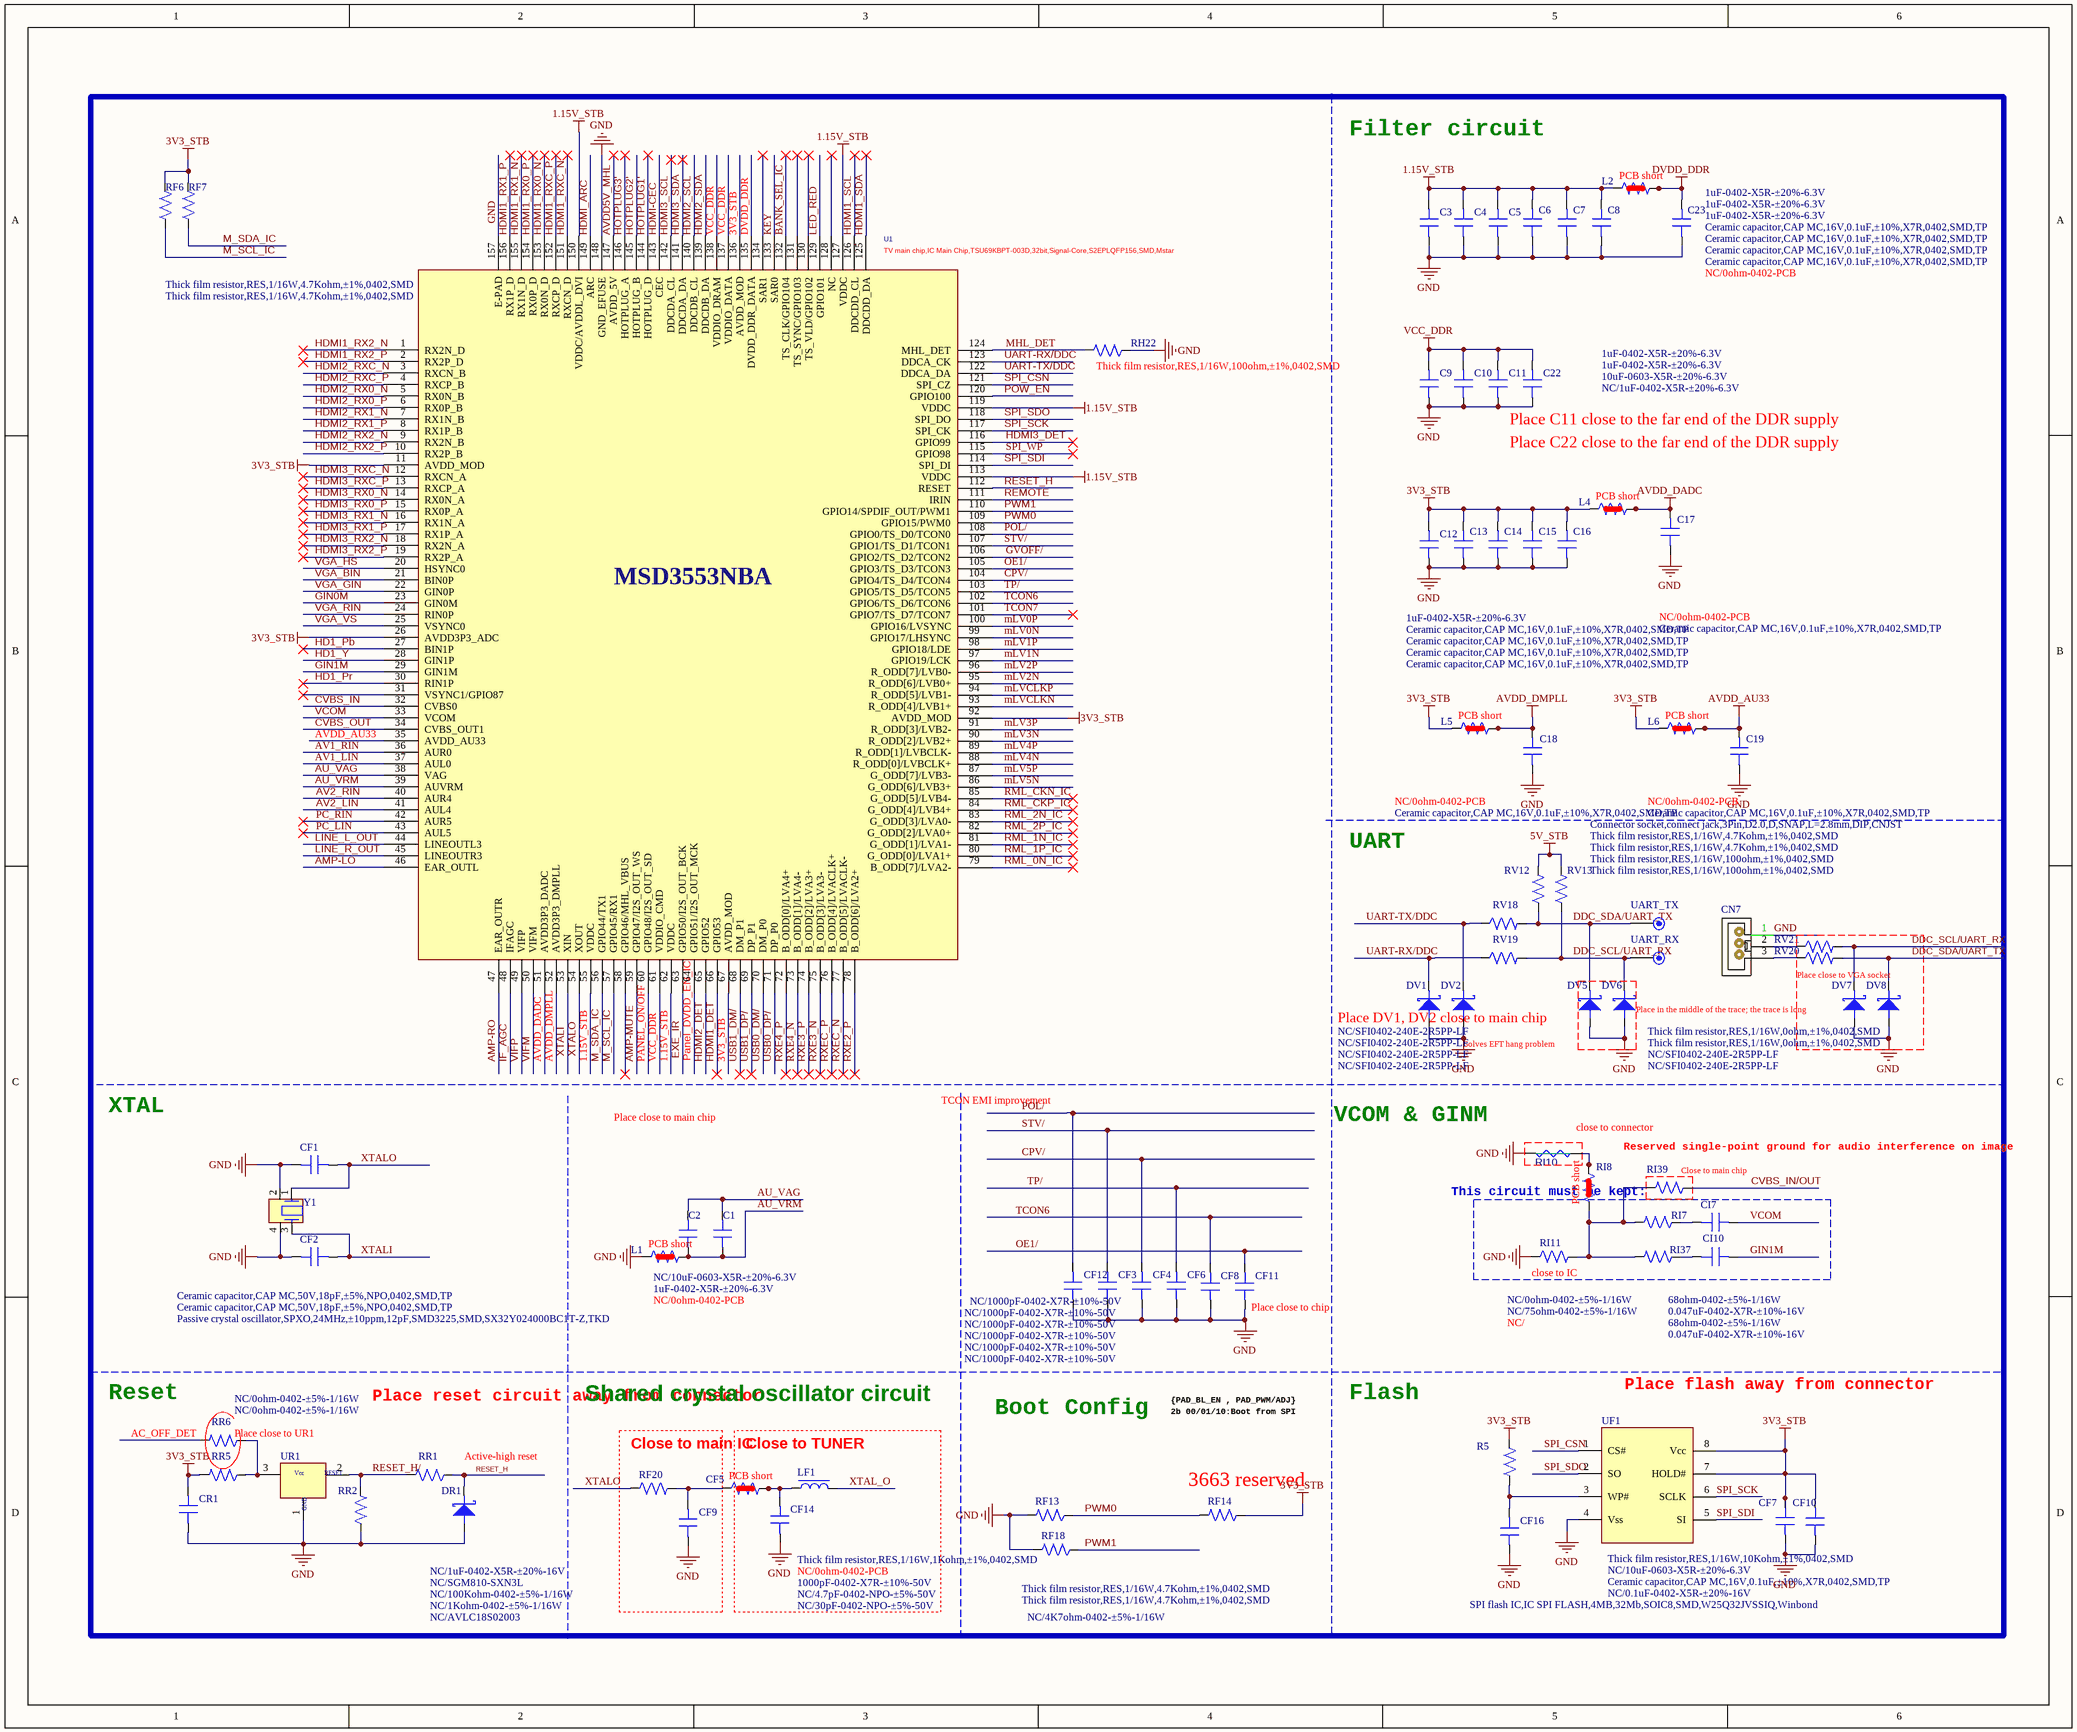
[diagram p0: MISC86383-12.SchDoc]
# Altium project MISC86383-33.PrjPCB (part 2 of 8)

## Sheet MISC86383-12.SchDoc
size 457 x 381 mm

### Parts
C1  1uF-0402-X5R-±20%-6.3V  [C0402]
C2  NC/10uF-0603-X5R-±20%-6.3V  [C0603]
C3  1uF-0402-X5R-±20%-6.3V  [C0402]
C4  1uF-0402-X5R-±20%-6.3V  [C0402]
C5  1uF-0402-X5R-±20%-6.3V  [C0402]
C6  Ceramic capacitor,CAP MC,16V,0.1uF,±10%,X7R,0402,SMD,TP  [C0402]
C7  Ceramic capacitor,CAP MC,16V,0.1uF,±10%,X7R,0402,SMD,TP  [C0402]
C8  Ceramic capacitor,CAP MC,16V,0.1uF,±10%,X7R,0402,SMD,TP  [C0402]
C9  1uF-0402-X5R-±20%-6.3V  [C0402]
C10  1uF-0402-X5R-±20%-6.3V  [C0402]
C11  10uF-0603-X5R-±20%-6.3V  [C0603]
C12  1uF-0402-X5R-±20%-6.3V  [C0402]
C13  Ceramic capacitor,CAP MC,16V,0.1uF,±10%,X7R,0402,SMD,TP  [C0402]
C14  Ceramic capacitor,CAP MC,16V,0.1uF,±10%,X7R,0402,SMD,TP  [C0402]
C15  Ceramic capacitor,CAP MC,16V,0.1uF,±10%,X7R,0402,SMD,TP  [C0402]
C16  Ceramic capacitor,CAP MC,16V,0.1uF,±10%,X7R,0402,SMD,TP  [C0402]
C17  Ceramic capacitor,CAP MC,16V,0.1uF,±10%,X7R,0402,SMD,TP  [C0402]
C18  Ceramic capacitor,CAP MC,16V,0.1uF,±10%,X7R,0402,SMD,TP  [C0402]
C19  Ceramic capacitor,CAP MC,16V,0.1uF,±10%,X7R,0402,SMD,TP  [C0402]
C22  NC/1uF-0402-X5R-±20%-6.3V  [C0402]
C23  Ceramic capacitor,CAP MC,16V,0.1uF,±10%,X7R,0402,SMD,TP  [C0402]
CF1  Ceramic capacitor,CAP MC,50V,18pF,±5%,NPO,0402,SMD,TP  [C0402]
CF2  Ceramic capacitor,CAP MC,50V,18pF,±5%,NPO,0402,SMD,TP  [C0402]
CF3  NC/1000pF-0402-X7R-±10%-50V  [C0402]
CF4  NC/1000pF-0402-X7R-±10%-50V  [C0402]
CF5  NC/0ohm-0402-PCB  [R0402SC]
CF6  NC/1000pF-0402-X7R-±10%-50V  [C0402]
CF7  Ceramic capacitor,CAP MC,16V,0.1uF,±10%,X7R,0402,SMD,TP  [C0402]
CF8  NC/1000pF-0402-X7R-±10%-50V  [C0402]
CF9  NC/30pF-0402-NPO-±5%-50V  [C0402]
CF10  NC/10uF-0603-X5R-±20%-6.3V  [C0603]
CF11  NC/1000pF-0402-X7R-±10%-50V  [C0402]
CF12  NC/1000pF-0402-X7R-±10%-50V  [C0402]
CF14  NC/4.7pF-0402-NPO-±5%-50V  [C0402]
CF16  NC/0.1uF-0402-X5R-±20%-16V  [C0402]
CI7  0.047uF-0402-X7R-±10%-16V  [C0402]
CI10  0.047uF-0402-X7R-±10%-16V  [C0402]
CN7  Connector socket,connect jack,3Pin,D2.0,D,SNAP,L=2.8mm,DIP,CNJST  [SIP3/2.0D-3]
CR1  NC/1uF-0402-X5R-±20%-16V  [C0402]
DR1  NC/AVLC18S02003  [DIODE-S0402]
DV1  NC/SFI0402-240E-2R5PP-LF  [DIODE-S0402]
DV2  NC/SFI0402-240E-2R5PP-LF  [DIODE-S0402]
DV5  NC/SFI0402-240E-2R5PP-LF  [DIODE-S0402]
DV6  NC/SFI0402-240E-2R5PP-LF  [DIODE-S0402]
DV7  NC/SFI0402-240E-2R5PP-LF  [DIODE-S0402]
DV8  NC/SFI0402-240E-2R5PP-LF  [DIODE-S0402]
L1  NC/0ohm-0402-PCB  [R0402SC]
L2  NC/0ohm-0402-PCB  [R0402SC]
L4  NC/0ohm-0402-PCB  [R0402SC]
L5  NC/0ohm-0402-PCB  [R0402SC]
L6  NC/0ohm-0402-PCB  [R0402SC]
LF1  1000pF-0402-X7R-±10%-50V  [L0402]
R5  Thick film resistor,RES,1/16W,10Kohm,±1%,0402,SMD  [R0402]
RF6  Thick film resistor,RES,1/16W,4.7Kohm,±1%,0402,SMD  [R0402]
RF7  Thick film resistor,RES,1/16W,4.7Kohm,±1%,0402,SMD  [R0402]
RF13  Thick film resistor,RES,1/16W,4.7Kohm,±1%,0402,SMD  [R0402]
RF14  NC/4K7ohm-0402-±5%-1/16W  [R0402]
RF18  Thick film resistor,RES,1/16W,4.7Kohm,±1%,0402,SMD  [R0402]
RF20  Thick film resistor,RES,1/16W,1Kohm,±1%,0402,SMD  [R0402]
RH22  Thick film resistor,RES,1/16W,100ohm,±1%,0402,SMD  [R0402]
RI7  68ohm-0402-±5%-1/16W  [R0402]
RI8  NC/  [R0402SC]
RI10  NC/SHORT  [GND]  (value not drawn)
RI11  NC/0ohm-0402-±5%-1/16W  [R0402]
RI37  68ohm-0402-±5%-1/16W  [R0402]
RI39  NC/75ohm-0402-±5%-1/16W  [R0402]
RR1  NC/1Kohm-0402-±5%-1/16W  [R0402]
RR2  NC/100Kohm-0402-±5%-1/16W  [R0402]
RR5  NC/0ohm-0402-±5%-1/16W  [R0402]
RR6  NC/0ohm-0402-±5%-1/16W  [R0402]
RV12  Thick film resistor,RES,1/16W,4.7Kohm,±1%,0402,SMD  [R0402]
RV13  Thick film resistor,RES,1/16W,4.7Kohm,±1%,0402,SMD  [R0402]
RV18  Thick film resistor,RES,1/16W,100ohm,±1%,0402,SMD  [R0402]
RV19  Thick film resistor,RES,1/16W,100ohm,±1%,0402,SMD  [R0402]
RV20  Thick film resistor,RES,1/16W,0ohm,±1%,0402,SMD  [R0402]
RV21  Thick film resistor,RES,1/16W,0ohm,±1%,0402,SMD  [R0402]
U1  TV main chip,IC Main Chip,TSU69KBPT-003D,32bit,Signal-Core,S2EPLQFP156,SMD,Mstar  [QFP156/0.4-2]
UART_RX  TEST  [TP]  (value not drawn)
UART_TX  TEST  [TP]  (value not drawn)
UF1  SPI flash IC,IC SPI FLASH,4MB,32Mb,SOIC8,SMD,W25Q32JVSSIQ,Winbond  [SOIC8]
UR1  NC/SGM810-SXN3L  [SO-23-1]
Y1  Passive crystal oscillator,SPXO,24MHz,±10ppm,12pF,SMD3225,SMD,SX32Y024000BC1T-Z,TKD  [XTAL-S-3]

### Blocks framed on the sheet
Place close to VGA socket: DV7 DV8 RV20 RV21
close to IC: CI7 CI10 RI7 RI11 RI37
Close to main IC: CF9 RF20
Close to TUNER: CF5 CF14 LF1

### Nets
1.15V_STB: C3.2 C4.2 C5.2 C6.2 C7.2 C8.2 L2.1 U1.55(VDDC) U1.62(VDDC) U1.113(VDDC) U1.119(VDDC) U1.127(VDDC) U1.150(VDDC/AVDDL_DVI)
3V3_STB: C12.2 C13.2 C14.2 C15.2 C16.2 CF7.1 CF10.2 CR1.2 L4.1 L5.1 L6.1 R5.2 RF6.2 RF7.2 RF14.1 RR5.2 U1.11(AVDD_MOD) U1.26(AVDD3P3_ADC) U1.67(AVDD_MOD) U1.92(AVDD_MOD) U1.136(AVDD_MOD) UF1.7(HOLD#) UF1.8(Vcc)
5V_STB: RV12.2 RV13.2
AVDD_AU33: C19.2 L6.2 L6.3 U1.35(AVDD_AU33)
AVDD_DADC: C17.2 L4.2 L4.3 U1.51(AVDD3P3_DADC)
AVDD_DMPLL: C18.2 L5.2 L5.3 U1.52(AVDD3P3_DMPLL)
DVDD_DDR: C23.2 L2.2 L2.3 U1.135(DVDD_DDR_DATA)
GND: C3.1 C4.1 C5.1 C6.1 C7.1 C8.1 C9.1 C10.1 C11.1 C12.1 C13.1 C14.1 C15.1 C16.1 C17.1 C18.1 C19.1 C22.1 C23.1 CF1.1 CF2.1 CF3.2 CF4.2 CF6.2 CF7.2 CF8.2 CF9.1 CF10.1 CF11.2 CF12.2 CF14.1 CF16.2 CN7.1 CR1.1 DR1.A DV1.A DV2.A DV5.A DV6.A DV7.A DV8.A L1.1 RF13.2 RF18.2 RH22.1 RI10.JP_1K RI11.1 RR2.2 U1.148(GND_EFUSE) U1.157(E-PAD) UF1.4(Vss) UR1.1(GND) Y1.2(G) Y1.4
VCC_DDR: C9.2 C10.2 C11.2 C22.2 U1.61(VDDIO_CMD) U1.137(VDDIO_DATA) U1.138(VDDIO_DRAM)
AC_OFF_DET: RR6.2
AMP-LO: U1.46(EAR_OUTL)
AMP-MUTE: U1.59(GPIO47/I2S_OUT_WS)
AMP-RO: U1.47(EAR_OUTR)
AU_VAG: C1.2 C2.2 U1.38(VAG)
AU_VRM: C1.1 C2.1 L1.2 L1.3 U1.39(AUVRM)
AV1_LIN: U1.37(AUL0)
AV1_RIN: U1.36(AUR0)
AV2_LIN: U1.41(AUL4)
AV2_RIN: U1.40(AUR4)
AVDD5V_MHL: U1.147(AVDD_5V)
BANK_SEL_IC: U1.132(TS_CLK/GPIO104)
CPV/: CF4.1 U1.104(GPIO4/TS_D4/TCON4)
CVBS_IN: U1.32(CVBS0)
CVBS_IN/OUT: RI39.1
CVBS_OUT: U1.34(CVBS_OUT1)
DDC_SCL/UART_RX: DV6.K DV7.K RV13.1 RV19.2 RV21.2 UART_RX.1
DDC_SDA/UART_TX: DV5.K DV8.K RV12.1 RV18.2 RV20.2 UART_TX.1
EXE_IR: U1.63(GPIO50/I2S_OUT_BCK)
GIN0M: U1.23(GIN0M)
GIN1M: CI10.1 U1.29(GIN1M)
GVOFF/: U1.106(GPIO2/TS_D2/TCON2)
HD1_Pb: U1.27(BIN1P)
HD1_Pr: U1.30(RIN1P)
HD1_Y: U1.28(GIN1P)
HDMI1_DET: U1.66(GPIO53)
HDMI1_RX0_N: U1.153(RX0N_D)
HDMI1_RX0_P: U1.154(RX0P_D)
HDMI1_RX1_N: U1.155(RX1N_D)
HDMI1_RX1_P: U1.156(RX1P_D)
HDMI1_RX2_N: U1.1(RX2N_D)
HDMI1_RX2_P: U1.2(RX2P_D)
HDMI1_RXC_N: U1.151(RXCN_D)
HDMI1_RXC_P: U1.152(RXCP_D)
HDMI1_SCL: U1.126(DDCDD_CL)
HDMI1_SDA: U1.125(DDCDD_DA)
HDMI2_DET: U1.65(GPIO52)
HDMI2_RX0_N: U1.5(RX0N_B)
HDMI2_RX0_P: U1.6(RX0P_B)
HDMI2_RX1_N: U1.7(RX1N_B)
HDMI2_RX1_P: U1.8(RX1P_B)
HDMI2_RX2_N: U1.9(RX2N_B)
HDMI2_RX2_P: U1.10(RX2P_B)
HDMI2_RXC_N: U1.3(RXCN_B)
HDMI2_RXC_P: U1.4(RXCP_B)
HDMI2_SCL: U1.140(DDCDB_CL)
HDMI2_SDA: U1.139(DDCDB_DA)
HDMI3_DET: U1.116(GPIO99)
HDMI3_RX0_N: U1.14(RX0N_A)
HDMI3_RX0_P: U1.15(RX0P_A)
HDMI3_RX1_N: U1.16(RX1N_A)
HDMI3_RX1_P: U1.17(RX1P_A)
HDMI3_RX2_N: U1.18(RX2N_A)
HDMI3_RX2_P: U1.19(RX2P_A)
HDMI3_RXC_N: U1.12(RXCN_A)
HDMI3_RXC_P: U1.13(RXCP_A)
HDMI3_SCL: U1.142(DDCDA_CL)
HDMI3_SDA: U1.141(DDCDA_DA)
HDMI-CEC: U1.143(CEC)
HDMI_ARC: U1.149(ARC)
HOTPLUG1': U1.144(HOTPLUG_D)
HOTPLUG2': U1.145(HOTPLUG_B)
HOTPLUG3': U1.146(HOTPLUG_A)
IF_AGC: U1.48(IFAGC)
KEY: U1.133(SAR0)
LED_RED: U1.129(GPIO101)
LINE_L_OUT: U1.44(LINEOUTL3)
LINE_R_OUT: U1.45(LINEOUTR3)
M_SCL_IC: RF6.1 U1.57(GPIO45/RX1)
M_SDA_IC: RF7.1 U1.56(GPIO44/TX1)
MHL_DET: RH22.2 U1.124(MHL_DET)
mLV0N: U1.99(GPIO17/LHSYNC)
mLV0P: U1.100(GPIO16/LVSYNC)
mLV1N: U1.97(GPIO19/LCK)
mLV1P: U1.98(GPIO18/LDE)
mLV2N: U1.95(R_ODD[6]/LVB0+)
mLV2P: U1.96(R_ODD[7]/LVB0-)
mLV3N: U1.90(R_ODD[2]/LVB2+)
mLV3P: U1.91(R_ODD[3]/LVB2-)
mLV4N: U1.88(R_ODD[0]/LVBCLK+)
mLV4P: U1.89(R_ODD[1]/LVBCLK-)
mLV5N: U1.86(G_ODD[6]/LVB3+)
mLV5P: U1.87(G_ODD[7]/LVB3-)
mLVCLKN: U1.93(R_ODD[4]/LVB1+)
mLVCLKP: U1.94(R_ODD[5]/LVB1-)
OE1/: CF11.1 U1.105(GPIO3/TS_D3/TCON3)
Panel_DVDD_EN_IC: U1.64(GPIO51/I2S_OUT_MCK)
PANEL_ON/OFF: U1.60(GPIO48/I2S_OUT_SD)
PC_LIN: U1.43(AUL5)
PC_RIN: U1.42(AUR5)
POL/: CF12.1 U1.108(GPIO0/TS_D0/TCON0)
POW_EN: U1.120(GPIO100)
PWM0: RF13.1 RF14.2 U1.109(GPIO15/PWM0)
PWM1: RF18.1 U1.110(GPIO14/SPDIF_OUT/PWM1)
REMOTE: U1.111(IRIN)
RESET_H: DR1.K RR1.1 U1.112(RESET)
RESET_H/: RR1.2 RR2.1 UR1.2(RESET)
RML_0N_IC: U1.79(B_ODD[7]/LVA2-)
RML_1N_IC: U1.81(G_ODD[1]/LVA1-)
RML_1P_IC: U1.80(G_ODD[0]/LVA1+)
RML_2N_IC: U1.83(G_ODD[3]/LVA0-)
RML_2P_IC: U1.82(G_ODD[2]/LVA0+)
RML_CKN_IC: U1.85(G_ODD[5]/LVB4-)
RML_CKP_IC: U1.84(G_ODD[4]/LVB4+)
RXE2_P: U1.78(B_ODD[6]/LVA2+)
RXE3_N: U1.75(B_ODD[3]/LVA3-)
RXE3_P: U1.74(B_ODD[2]/LVA3+)
RXE4_N: U1.73(B_ODD[1]/LVA4-)
RXE4_P: U1.72(B_ODD[0]/LVA4+)
RXEC_N: U1.77(B_ODD[5]/LVACLK-)
RXEC_P: U1.76(B_ODD[4]/LVACLK+)
SPI_CSN: U1.121(SPI_CZ) UF1.1(CS#)
SPI_SCK: U1.117(SPI_CK) UF1.6(SCLK)
SPI_SDI: U1.114(SPI_DI) UF1.5(SI)
SPI_SDO: U1.118(SPI_DO) UF1.2(SO)
SPI_WP: U1.115(GPIO98)
STV/: CF3.1 U1.107(GPIO1/TS_D1/TCON1)
TCON6: CF8.1 U1.102(GPIO6/TS_D6/TCON6)
TCON7: U1.101(GPIO7/TS_D7/TCON7)
TP/: CF6.1 U1.103(GPIO5/TS_D5/TCON5)
UART-RX/DDC: DV1.K RV19.1 U1.123(DDCA_CK)
UART-TX/DDC: DV2.K RV18.1 U1.122(DDCA_DA)
USB0_DM/: U1.70(DM_P0)
USB0_DP/: U1.71(DP_P0)
USB1_DM/: U1.68(DM_P1)
USB1_DP/: U1.69(DP_P1)
VCOM: CI7.1 U1.33(VCOM)
VGA_BIN: U1.21(BIN0P)
VGA_GIN: U1.22(GIN0P)
VGA_HS: U1.20(HSYNC0)
VGA_RIN: U1.24(RIN0P)
VGA_VS: U1.25(VSYNC0)
VIFM: U1.50(VIFM)
VIFP: U1.49(VIFP)
XTAL_O: LF1.2
XTALI: CF2.2 U1.53(XIN) Y1.3
XTALO: CF1.2 RF20.1 U1.54(XOUT) Y1.1
NetCF5_1: CF5.1 CF9.2 RF20.2
NetCF5_2: CF5.2 CF5.3 CF14.2 LF1.1
NetCF16_1: CF16.1 R5.1 UF1.3(WP#)
NetCI7_2: CI7.2 RI7.1
NetCI10_2: CI10.2 RI37.1
NetCN7_2: CN7.2 RV21.1
NetCN7_3: CN7.3 RV20.1
NetRI7_2: RI7.2 RI8.1 RI11.2 RI37.2 RI39.2
NetRI8_2: RI8.2 RI8.3 RI10.JP_2K
NetRR5_1: RR5.1 RR6.1 UR1.3(Vcc)

Not connected (* = marked no-connect by the designer): U1 31(VSYNC1/GPIO87)* 58(GPIO46/MHL_VBUS)* 128(NC)* 130(TS_VLD/GPIO102)* 131(TS_SYNC/GPIO103)* 134(SAR1)*

### Notes on the sheet
- Filter circuit
- Place C11 close to the far end of the DDR supply
- Place C22 close to the far end of the DDR supply
- UART
- Place DV1, DV2 close to main chip
- (near DV2) Solves EFT hang problem
- Place in the middle of the trace; the trace is long
- XTAL
- TCON EMI improvement
- Place close to main chip
- VCOM & GINM
- (near RI10) close to connector
- Reserved single-point ground for audio interference on image
- (near RI39) Close to main chip
- (near RI8) This circuit must be kept:
- (near CF11) Place close to chip
- Reset
- Place reset circuit away from connector
- Shared crystal oscillator circuit
- {PAD_BL_EN , PAD_PWM/ADJ}
- Flash
- Place flash away from connector
- (near RR6) Place close to UR1
- Active-high reset
- Boot Config
- 2b 00/01/10:Boot from SPI
- (near RF14) 3663 reserved

### Library data of the parts
C1 = 2.2uF-0402-X5R-±20%-6.3V-D
C2 C11 CF10 = 10uF-0603-X5R-±20%-6.3V-D
C3-C5 C9 C10 C12 C22 CR1 = 1uF-0402-X5R-±20%-6.3V-D
C6-C8 C13-C19 C23 CF7 CF16 = 0.1uF-0402-Y5V-+80%-20%-16V-D
CF1 CF2 = 004.003.0000527-D: Ceramic capacitor,CAP MC,50V,18pF,±5%,NPO,0402,SMD,TP-D
CF3 CF4 CF6 CF8 CF11 CF12 = 1000pF-0402-X7R-±10%-50V-D
CF5 L1 L2 L4-L6 RI8 = 0ohm-0402-PCB-D
CF9 CF14 = 30pF-0402-NPO-±5%-50V-D
CI7 CI10 = 0.047uF-0402-X7R-±10%-16V-D
CN7 = 3PIN-2.0-D-H-G-带扣-DHMI
DR1 DV1 DV2 DV5-DV8 = AVLC18S02003-D
LF1 = MGHB1005S102T-LF-D
R5 = 10Kohm-0402-±5%-1/16W-D
RF6 RF7 RF13 RF14 RF18 RV12 RV13 = 4K7ohm-0402-±5%-1/16W-D
RF20 = 220ohm-0402-±5%-1/16W-D
RH22 = 300Kohm-0402-±5%-1/16W-D
RI7 RI37 = 68ohm-0402-±5%-1/16W-D
RI10 = GND: Manufacturer: Panasonic; Part Number: ERJ3GEYJ473V; Right: 20; Bottom: 30; CLASS: Discrete; Comments: Digikey
RI11 = 0ohm-0402-±5%-1/16W-D
RI39 = 75ohm-0402-±5%-1/16W-D
RR1 RR5 RR6 = 1Kohm-0402-±5%-1/16W-D
RR2 = 100Kohm-0402-±5%-1/16W-D
RV18-RV21 = 100ohm-0402-±5%-1/16W-D
U1 = TV主芯片,IC Main Chip,MSD3553NBCT-005X,32bit,Single-Core,EpLQFP156,SMD,Mstar-D: PCB DECAL: IC-156P-EPLQFP; Source_Path: WHISKY SCH20150520C.DSN
UF1 = SPI FLASH 芯片,IC SPI FLASH,64Mb,SOIC8,SMD,GD25Q64CSIG,GigaDevice-D
UR1 = SGM810-SXN3L-D
Y1 = 32MHz-±10PPM-12PF-SMD3225-JWT-D